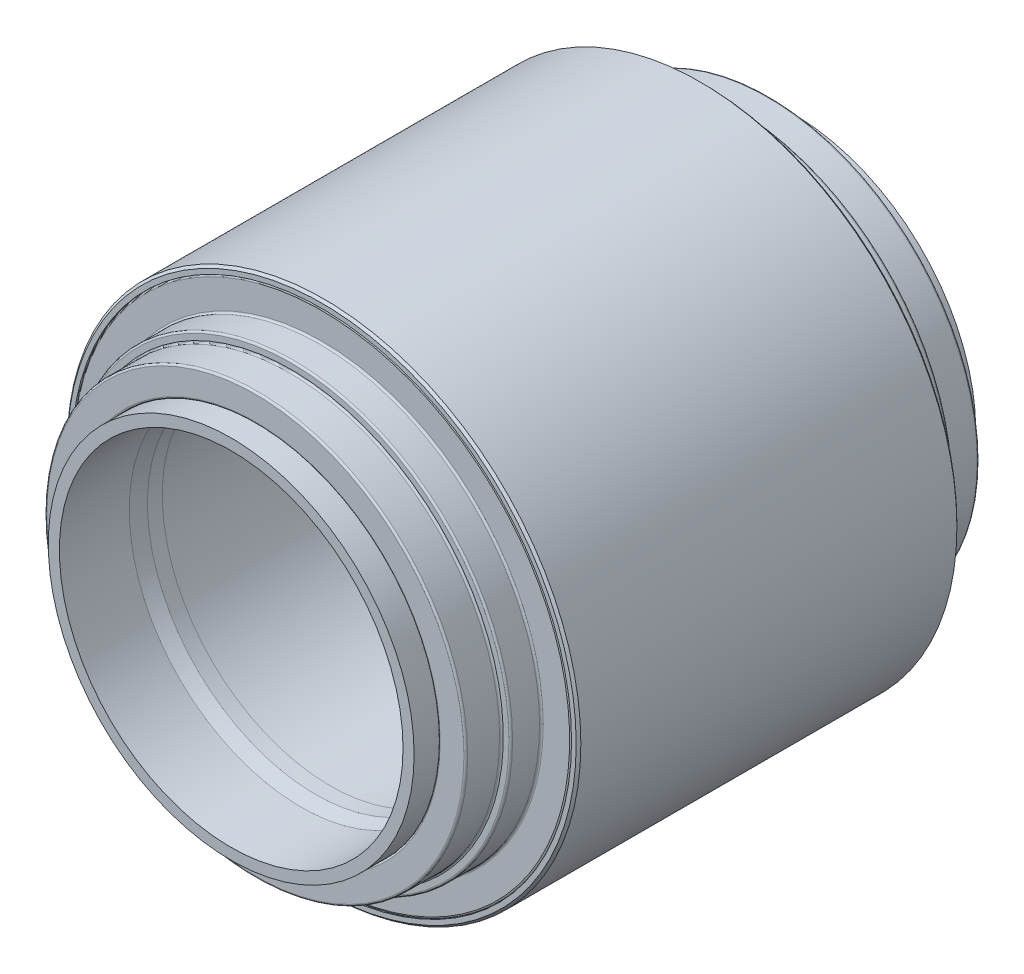
SolidWorks part; units mm, degrees
material "普通碳钢"
ref_plane "Front Plane" through (0, 0, 0) normal (0, 0, 1) x (1, 0, 0)
ref_plane "Top Plane" through (0, 0, 0) normal (0, 1, 0) x (1, 0, 0)
ref_plane "Right Plane" through (0, 0, 0) normal (1, 0, 0) x (0, 0, -1)
sketch "Sketch1" plane through (0, 0, 0) normal (1, 0, 0) x (0, 0, -1)
  line L0 (-191.0635, 0) -> (0, 0) construction
  line L1 (0, 0) -> (0, 192.8904) construction
  line L2 (81.756, 110.331) -> (-81.756, 110.331)
  line L3 (-81.756, 110.331) -> (-81.756, 94.385)
  line L4 (-68.596, 107.331) -> (-68.596, 105.831)
  line L5 (84.33, 72.225) -> (-84.33, 72.225)
  line L6 (-70.9191, 83.7968) -> (-66.7213, 105.3926)
  line L7 (-81.756, 107.331) -> (-68.596, 107.331)
  line L8 (-68.596, 105.831) -> (-18, 94)
  line L9 (-15, 72.225) -> (-15, 80.225)
  line L10 (-15, 77.225) -> (15, 77.225)
  line L11 (-15, 80.225) -> (-20.6776, 80.225)
  line L12 (-120.6, 73.8) -> (-120.6, 78.575)
  line L13 (-21.4777, 76.1086) -> (-70.9191, 83.7968)
  line L14 (-120.6, 73.8) -> (-90.6, 73.8)
  line L15 (-70.2528, 87.225) -> (-77.98, 87.225)
  line L16 (-87.98, 78.575) -> (-77.98, 77.7001)
  line L17 (-21.4777, 76.1086) -> (-18, 94)
  line L18 (-18, 94) -> (18, 94)
  line L19 (-19.7389, 85.0543) -> (-68.8202, 94.5947) construction
  line L20 (-120.6, 78.575) -> (-87.98, 78.575)
  line L21 (-68.596, 105.831) -> (-80.256, 105.831)
  line L22 (-90.6, 73.8) -> (-84.33, 72.225)
  line L23 (-77.98, 72.225) -> (-77.98, 87.225)
  line L24 (-81.756, 94.385) -> (-94.916, 94.385)
  line L25 (-94.916, 94.385) -> (-94.916, 90.385)
  line L26 (-94.916, 90.385) -> (-110.226, 90.385)
  line L27 (-110.226, 90.385) -> (-110.226, 78.575)
  line L28 (80.256, 92.885) -> (80.256, 105.831)
  line L29 (-108.726, 78.575) -> (-108.726, 88.885)
  line L30 (-108.726, 88.885) -> (-93.416, 88.885)
  line L31 (-93.416, 78.575) -> (-93.416, 92.885)
  line L32 (-93.416, 92.885) -> (-80.256, 92.885)
  line L33 (-80.256, 92.885) -> (-80.256, 105.831)
  line L34 (93.416, 92.885) -> (80.256, 92.885)
  line L35 (93.416, 78.575) -> (93.416, 92.885)
  line L36 (108.726, 88.885) -> (93.416, 88.885)
  line L37 (108.726, 78.575) -> (108.726, 88.885)
  line L38 (110.226, 90.385) -> (110.226, 78.575)
  line L39 (94.916, 90.385) -> (110.226, 90.385)
  line L40 (94.916, 94.385) -> (94.916, 90.385)
  line L41 (81.756, 94.385) -> (94.916, 94.385)
  line L42 (77.98, 72.225) -> (77.98, 87.225)
  line L43 (90.6, 73.8) -> (84.33, 72.225)
  line L44 (68.596, 105.831) -> (80.256, 105.831)
  line L45 (120.6, 78.575) -> (87.98, 78.575)
  line L46 (21.4777, 76.1086) -> (18, 94)
  line L47 (87.98, 78.575) -> (77.98, 77.7001)
  line L48 (70.2528, 87.225) -> (77.98, 87.225)
  line L49 (120.6, 73.8) -> (90.6, 73.8)
  line L50 (21.4777, 76.1086) -> (70.9191, 83.7968)
  line L51 (120.6, 73.8) -> (120.6, 78.575)
  line L52 (15, 80.225) -> (20.6776, 80.225)
  line L53 (15, 72.225) -> (15, 80.225)
  line L54 (68.596, 105.831) -> (18, 94)
  line L55 (81.756, 107.331) -> (68.596, 107.331)
  line L56 (70.9191, 83.7968) -> (66.7213, 105.3926)
  line L57 (68.596, 107.331) -> (68.596, 105.831)
  line L58 (81.756, 110.331) -> (81.756, 94.385)
  point P63 (0, 94)
  point P71 (0, 77.225)
  point P75 (0, 72.225)
  point P76 (0, 110.331)
  dimension "D1" = 220.662
  dimension "D2" = 163.512
  dimension "D3" = 3
  dimension "D4" = 11
  dimension "D5" = 1.5
  dimension "D6" = 1.5
  dimension "D7" = 22
  dimension "D8" = 144.45
  dimension "D9" = 15
  dimension "D10" = 5
  dimension "D11" = 5
  dimension "D12" = 50
  dimension "D13" = 15
  dimension "D14" = 188
  dimension "D15" = 18
  dimension "D16" = 120.6
  dimension "D17" = 10
  dimension "D18" = 3
  dimension "D19" = 157.15
  dimension "D20" = 147.6
  dimension "D21" = 42.62
  dimension "D22" = 6.35
  dimension "D23" = 188.77
  dimension "D24" = 41.63
  dimension "D25" = 1.5
  dimension "D26" = 1.5
  dimension "D27" = 1.5
  dimension "D28" = 1.5
  dimension "D29" = 13.16
  dimension "D30" = 13.16
  dimension "D31" = 4
  dimension "D32" = 30
ref_plane "Plane1" through (0, 0, 0) normal (0.9927, -0.1205, 0) x (0, 0, -1)
sketch "Sketch2" plane through (0, 0, 0) normal (1, 0, 0) x (0, 0, -1)
  line L0 (15, 72.225) -> (15, 80.225) construction
  line L1 (84.33, 72.225) -> (-84.33, 72.225) construction
  line L2 (-15, 72.225) -> (-15, 80.225) construction
  line L3 (-15, 77.225) -> (15, 77.225) construction
  line L4 (15, 72.225) -> (15, 77.225)
  line L5 (15, 72.225) -> (-15, 72.225)
  line L6 (-15, 72.225) -> (-15, 77.225)
  line L7 (-15, 77.225) -> (15, 77.225)
  line L8 (-191.0635, 0) -> (0, 0) construction
revolve "Revolve1" add sketch "Sketch2" angle 360 about L8
sketch "Sketch3" plane through (0, 0, 0) normal (1, 0, 0) x (0, 0, -1)
  line L0 (-21.4777, 76.1086) -> (-70.9191, 83.7968) construction
  line L1 (-70.9191, 83.7968) -> (-66.7213, 105.3926) construction
  line L2 (-70.2528, 87.225) -> (-77.98, 87.225) construction
  line L3 (-77.98, 72.225) -> (-77.98, 87.225) construction
  line L4 (84.33, 72.225) -> (-84.33, 72.225) construction
  line L5 (-15, 72.225) -> (-15, 80.225) construction
  line L6 (-15, 80.225) -> (-20.6776, 80.225) construction
  line L7 (-21.4777, 76.1086) -> (-18, 94) construction
  line L8 (-21.4777, 76.1086) -> (-70.9191, 83.7968)
  line L9 (-70.9191, 83.7968) -> (-70.2528, 87.225)
  line L10 (-70.2528, 87.225) -> (-77.98, 87.225)
  line L11 (-77.98, 72.225) -> (-77.98, 87.225)
  line L12 (-15, 72.225) -> (-77.98, 72.225)
  line L13 (-15, 72.225) -> (-15, 80.225)
  line L14 (-15, 80.225) -> (-20.6776, 80.225)
  line L15 (-21.4777, 76.1086) -> (-20.6776, 80.225)
  line L16 (-191.0635, 0) -> (0, 0) construction
revolve "Revolve2" add sketch "Sketch3" angle 360 about L16
sketch "Sketch4" plane through (0, 0, 0) normal (1, 0, 0) x (0, 0, -1)
  line L0 (-77.98, 72.225) -> (-77.98, 87.225) construction
  line L1 (-120.6, 73.8) -> (-120.6, 78.575) construction
  line L2 (-120.6, 78.575) -> (-87.98, 78.575) construction
  line L3 (-87.98, 78.575) -> (-77.98, 77.7001) construction
  line L4 (-120.6, 73.8) -> (-90.6, 73.8) construction
  line L5 (-90.6, 73.8) -> (-84.33, 72.225) construction
  line L6 (84.33, 72.225) -> (-84.33, 72.225) construction
  line L7 (-77.98, 72.225) -> (-77.98, 77.7001)
  line L8 (-120.6, 73.8) -> (-120.6, 78.575)
  line L9 (-120.6, 78.575) -> (-87.98, 78.575)
  line L10 (-87.98, 78.575) -> (-77.98, 77.7001)
  line L11 (-120.6, 73.8) -> (-90.6, 73.8)
  line L12 (-90.6, 73.8) -> (-84.33, 72.225)
  line L13 (-77.98, 72.225) -> (-84.33, 72.225)
  line L14 (-191.0635, 0) -> (0, 0) construction
revolve "Revolve3" add sketch "Sketch4" angle 360 about L14
sketch "Sketch5" plane through (0, 0, 0) normal (1, 0, 0) x (0, 0, -1)
  line L0 (-108.726, 78.575) -> (-108.726, 88.885) construction
  line L1 (-108.726, 88.885) -> (-93.416, 88.885) construction
  line L2 (-93.416, 78.575) -> (-93.416, 92.885) construction
  line L3 (-120.6, 78.575) -> (-87.98, 78.575) construction
  line L4 (-108.726, 78.575) -> (-108.726, 88.885)
  line L5 (-108.726, 88.885) -> (-93.416, 88.885)
  line L6 (-93.416, 78.575) -> (-93.416, 88.885)
  line L7 (-108.726, 78.575) -> (-93.416, 78.575)
  line L8 (-191.0635, 0) -> (0, 0) construction
revolve "Revolve4" add sketch "Sketch5" angle 360 about L8
sketch "Sketch6" plane through (0, 0, 0) normal (1, 0, 0) x (0, 0, -1)
  line L0 (-68.596, 107.331) -> (-68.596, 105.831) construction
  line L1 (-81.756, 110.331) -> (-81.756, 94.385) construction
  line L2 (-68.596, 105.831) -> (-80.256, 105.831) construction
  line L3 (-81.756, 107.331) -> (-68.596, 107.331) construction
  line L4 (-80.256, 92.885) -> (-80.256, 105.831) construction
  line L5 (-81.756, 94.385) -> (-94.916, 94.385) construction
  line L6 (-93.416, 92.885) -> (-80.256, 92.885) construction
  line L7 (-93.416, 78.575) -> (-93.416, 92.885) construction
  line L8 (-94.916, 94.385) -> (-94.916, 90.385) construction
  line L9 (-94.916, 90.385) -> (-110.226, 90.385) construction
  line L10 (-108.726, 88.885) -> (-93.416, 88.885) construction
  line L11 (-108.726, 78.575) -> (-108.726, 88.885) construction
  line L12 (-120.6, 78.575) -> (-87.98, 78.575) construction
  line L13 (-110.226, 90.385) -> (-110.226, 78.575) construction
  line L14 (-68.596, 107.331) -> (-68.596, 105.831)
  line L15 (-81.756, 107.331) -> (-81.756, 94.385)
  line L16 (-68.596, 105.831) -> (-80.256, 105.831)
  line L17 (-81.756, 107.331) -> (-68.596, 107.331)
  line L18 (-80.256, 92.885) -> (-80.256, 105.831)
  line L19 (-81.756, 94.385) -> (-94.916, 94.385)
  line L20 (-93.416, 92.885) -> (-80.256, 92.885)
  line L21 (-93.416, 88.885) -> (-93.416, 92.885)
  line L22 (-94.916, 94.385) -> (-94.916, 90.385)
  line L23 (-94.916, 90.385) -> (-110.226, 90.385)
  line L24 (-108.726, 88.885) -> (-93.416, 88.885)
  line L25 (-108.726, 78.575) -> (-108.726, 88.885)
  line L26 (-110.226, 78.575) -> (-108.726, 78.575)
  line L27 (-110.226, 90.385) -> (-110.226, 78.575)
  line L28 (-191.0635, 0) -> (0, 0) construction
revolve "Revolve5" add sketch "Sketch6" angle 360 about L28
sketch "Sketch7" plane through (0, 0, 0) normal (-0.9927, 0.1205, 0) x (0, 0, -1)
  line L8 (-68.8202, 94.5947) -> (-14.2013, 83.9779) construction
  line L9 (-66.7205, 105.3914) -> (-18.0012, 93.9992)
  line L10 (-19.7397, 85.0555) -> (-18.0012, 93.9992)
  line L11 (-19.7397, 85.0555) -> (-68.8191, 94.5955)
  line L12 (-68.8191, 94.5955) -> (-66.7205, 105.3914)
revolve "Revolve7" add sketch "Sketch7" angle 360 about L8
sketch "Sketch9" plane through (0, 0, 0) normal (1, 0, 0) x (0, 0, -1)
  line L0 (-191.0635, 0) -> (0, 0) construction
  line L1 (70.9191, 83.7968) -> (66.7213, 105.3926) construction
  line L2 (70.2528, 87.225) -> (77.98, 87.225) construction
  line L3 (77.98, 72.225) -> (77.98, 87.225) construction
  line L4 (84.33, 72.225) -> (-84.33, 72.225) construction
  line L5 (15, 72.225) -> (15, 80.225) construction
  line L6 (15, 80.225) -> (20.6776, 80.225) construction
  line L7 (21.4777, 76.1086) -> (18, 94) construction
  line L8 (21.4777, 76.1086) -> (70.9191, 83.7968) construction
  line L9 (70.9191, 83.7968) -> (70.2528, 87.225)
  line L10 (70.2528, 87.225) -> (77.98, 87.225)
  line L11 (77.98, 72.225) -> (77.98, 87.225)
  line L12 (77.98, 72.225) -> (15, 72.225)
  line L13 (15, 72.225) -> (15, 80.225)
  line L14 (15, 80.225) -> (20.6776, 80.225)
  line L15 (21.4777, 76.1086) -> (20.6776, 80.225)
  line L16 (21.4777, 76.1086) -> (70.9191, 83.7968)
revolve "Revolve9" add sketch "Sketch9" angle 360 about L0
sketch "Sketch10" plane through (0, 0, 0) normal (1, 0, 0) x (0, 0, -1)
  line L0 (90.6, 73.8) -> (84.33, 72.225) construction
  line L1 (84.33, 72.225) -> (-84.33, 72.225) construction
  line L2 (77.98, 72.225) -> (77.98, 87.225) construction
  line L3 (87.98, 78.575) -> (77.98, 77.7001) construction
  line L4 (120.6, 78.575) -> (87.98, 78.575) construction
  line L5 (120.6, 73.8) -> (120.6, 78.575) construction
  line L6 (120.6, 73.8) -> (90.6, 73.8) construction
  line L7 (90.6, 73.8) -> (84.33, 72.225)
  line L8 (84.33, 72.225) -> (77.98, 72.225)
  line L9 (77.98, 72.225) -> (77.98, 77.7001)
  line L10 (87.98, 78.575) -> (77.98, 77.7001)
  line L11 (120.6, 78.575) -> (87.98, 78.575)
  line L12 (120.6, 73.8) -> (120.6, 78.575)
  line L13 (120.6, 73.8) -> (90.6, 73.8)
  line L14 (-191.0635, 0) -> (0, 0) construction
revolve "Revolve10" add sketch "Sketch10" angle 360 about L14
sketch "Sketch11" plane through (0, 0, 0) normal (1, 0, 0) x (0, 0, -1)
  line L0 (108.726, 78.575) -> (108.726, 88.885) construction
  line L1 (120.6, 78.575) -> (87.98, 78.575) construction
  line L2 (108.726, 88.885) -> (93.416, 88.885) construction
  line L3 (93.416, 78.575) -> (93.416, 92.885) construction
  line L4 (108.726, 78.575) -> (108.726, 88.885)
  line L5 (108.726, 78.575) -> (93.416, 78.575)
  line L6 (108.726, 88.885) -> (93.416, 88.885)
  line L7 (93.416, 78.575) -> (93.416, 88.885)
  line L8 (-191.0635, 0) -> (0, 0) construction
revolve "Revolve11" add sketch "Sketch11" angle 360 about L8
sketch "Sketch12" plane through (0, 0, 0) normal (1, 0, 0) x (0, 0, -1)
  line L0 (120.6, 78.575) -> (87.98, 78.575) construction
  line L1 (110.226, 90.385) -> (110.226, 78.575) construction
  line L2 (108.726, 78.575) -> (108.726, 88.885) construction
  line L3 (108.726, 88.885) -> (93.416, 88.885) construction
  line L4 (93.416, 78.575) -> (93.416, 92.885) construction
  line L5 (94.916, 94.385) -> (94.916, 90.385) construction
  line L6 (94.916, 90.385) -> (110.226, 90.385) construction
  line L7 (81.756, 94.385) -> (94.916, 94.385) construction
  line L8 (93.416, 92.885) -> (80.256, 92.885) construction
  line L9 (81.756, 110.331) -> (81.756, 94.385) construction
  line L10 (80.256, 92.885) -> (80.256, 105.831) construction
  line L11 (68.596, 105.831) -> (80.256, 105.831) construction
  line L12 (68.596, 107.331) -> (68.596, 105.831) construction
  line L13 (81.756, 107.331) -> (68.596, 107.331) construction
  line L14 (110.226, 78.575) -> (108.726, 78.575)
  line L15 (110.226, 90.385) -> (110.226, 78.575)
  line L16 (108.726, 78.575) -> (108.726, 88.885)
  line L17 (108.726, 88.885) -> (93.416, 88.885)
  line L18 (93.416, 88.885) -> (93.416, 92.885)
  line L19 (94.916, 94.385) -> (94.916, 90.385)
  line L20 (94.916, 90.385) -> (110.226, 90.385)
  line L21 (81.756, 94.385) -> (94.916, 94.385)
  line L22 (93.416, 92.885) -> (80.256, 92.885)
  line L23 (81.756, 107.331) -> (81.756, 94.385)
  line L24 (80.256, 92.885) -> (80.256, 105.831)
  line L25 (68.596, 105.831) -> (80.256, 105.831)
  line L26 (68.596, 107.331) -> (68.596, 105.831)
  line L27 (81.756, 107.331) -> (68.596, 107.331)
  line L28 (0, 0) -> (-191.0635, 0) construction
revolve "Revolve12" add sketch "Sketch12" angle 360 about L28
sketch "Sketch13" plane through (0, 0, 0) normal (-0.9927, 0.1205, 0) x (0, 0, -1)
  line L3 (21.4777, -75.5537) -> (18, -93.3146) construction
  line L5 (18.0008, -93.3159) -> (19.7399, -84.4344)
  line L6 (19.7399, -84.4344) -> (68.8359, -93.8304)
  line L7 (66.7221, -104.6254) -> (68.8359, -93.8304)
  line L8 (70.9191, -83.1859) -> (66.7213, -104.6242) construction
  line L9 (19.7389, -84.4342) -> (68.8359, -93.8304) construction
  line L10 (66.7221, -104.6254) -> (18.0008, -93.3159)
  line L12 (68.596, -105.0594) -> (18, -93.3146) construction
  dimension "D2" = 0.001
  dimension "D3" = 0.001
  dimension "D4" = 11
  dimension "D5" = 0.001
revolve "Revolve13" add sketch "Sketch13" angle 360 about L6
sketch "Sketch8" plane through (0, 0, 0) normal (1, 0, 0) x (0, 0, -1)
  line L0 (-68.596, 107.331) -> (-68.596, 105.831) construction
  line L1 (68.596, 107.331) -> (68.596, 105.831) construction
  line L2 (81.756, 110.331) -> (81.756, 94.385) construction
  line L3 (81.756, 107.331) -> (68.596, 107.331) construction
  line L4 (81.756, 110.331) -> (-81.756, 110.331) construction
  line L5 (-81.756, 107.331) -> (-68.596, 107.331) construction
  line L6 (-68.596, 105.831) -> (-18, 94) construction
  line L7 (-18, 94) -> (18, 94) construction
  line L8 (68.596, 105.831) -> (18, 94) construction
  line L9 (-68.596, 107.331) -> (-68.596, 105.831)
  line L10 (68.596, 107.331) -> (68.596, 105.831)
  line L11 (81.756, 110.331) -> (81.756, 107.331)
  line L12 (81.756, 107.331) -> (68.596, 107.331)
  line L13 (81.756, 110.331) -> (-81.756, 110.331)
  line L14 (-81.756, 107.331) -> (-68.596, 107.331)
  line L15 (-68.596, 105.831) -> (-18, 94)
  line L16 (-18, 94) -> (18, 94)
  line L17 (68.596, 105.831) -> (18, 94)
  line L18 (-81.756, 110.331) -> (-81.756, 94.385) construction
  line L19 (-81.756, 110.331) -> (-81.756, 107.331)
  line L20 (-191.0635, 0) -> (0, 0) construction
revolve "Revolve8" add sketch "Sketch8" angle 360 about L20
fillet "Fillet1" radius 0.8 6 edges at (107.331, 0, 81.756) (90.385, 0, 110.226) (78.575, 0, 110.226) (94.385, 0, 94.916) (90.385, 0, 94.916) (94.385, 0, 81.756)
fillet "Fillet2" radius 0.8 6 edges at (-94.385, 0, -81.756) (-107.331, 0, -81.756) (-78.575, 0, -110.226) (-90.385, 0, -110.226) (-90.385, 0, -94.916) (-94.385, 0, -94.916)
chamfer "Chamfer1" distance 1 angle 45 2 edges at (110.331, 0, -81.756) (110.331, 0, 81.756)
pattern_circular "CirPattern5" count 26 over 360 about axis through (0, 0, 0) along (0, 0, 1) of "Revolve7"
pattern_circular "CirPattern7" count 26 over 360 about axis through (0, 0, 191.0635) along (0, 0, -1) of "Revolve13"
sketch "Sketch14" plane through (0, 0, 0) normal (0, 1, 0) x (1, 0, 0)
  line L0 (0, 0) -> (0, 147.1956) construction
  line L1 (78.575, 120.6) -> (-78.575, 120.6) construction
  circle A0 centre (0, 120.6) radius 3
  dimension "D1" = 6
extrude "Cut-Extrude1" cut sketch "Sketch14" along normal through all
